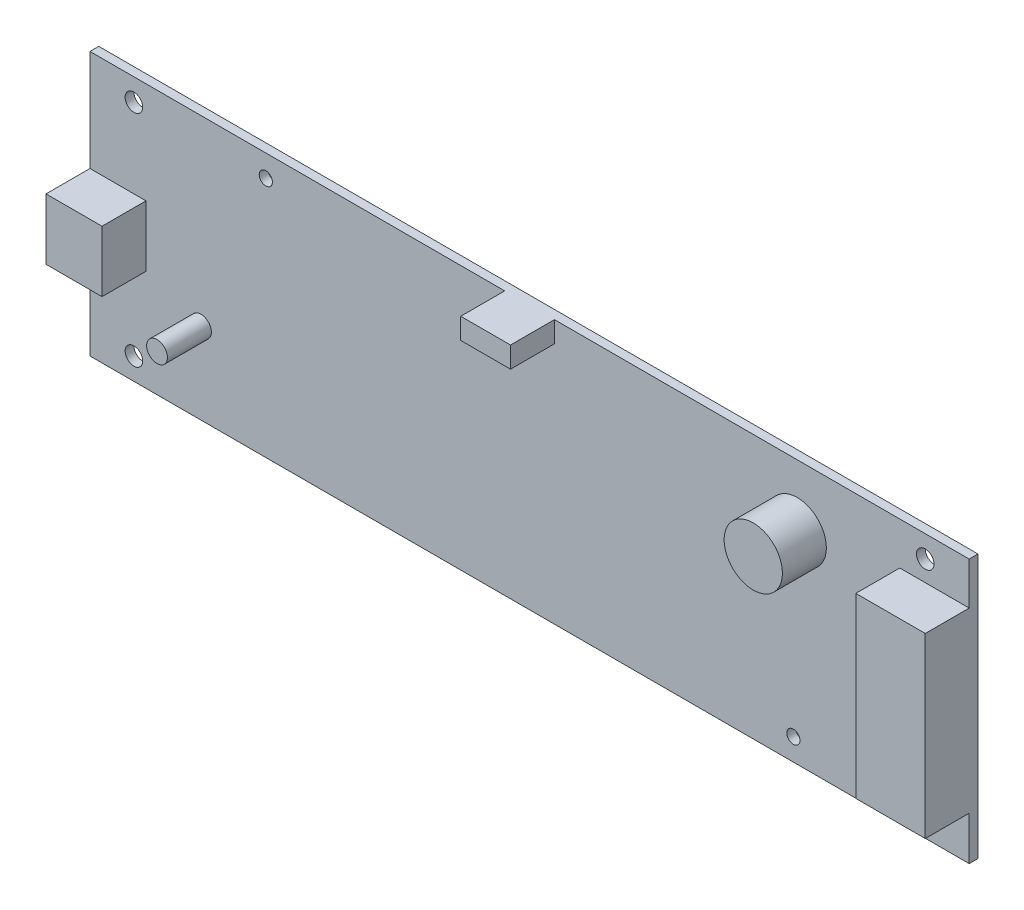
SolidWorks part; units mm, degrees
ref_plane "Front Plane" through (0, 0, 0) normal (0, 0, 1) x (1, 0, 0)
ref_plane "Top Plane" through (0, 0, 0) normal (0, 1, 0) x (1, 0, 0)
ref_plane "Right Plane" through (0, 0, 0) normal (1, 0, 0) x (0, 0, -1)
other "Configuration Table"
sketch "Sketch1" plane through (0, 0, 0) normal (0, 0, 1) x (1, 0, 0)
  line L1 (-50, 15) -> (50, 15)
  line L2 (-50, 15) -> (-50, -15)
  line L3 (-50, -15) -> (50, -15)
  line L4 (50, 15) -> (50, -15)
  line L5 (-50, 15) -> (50, -15) construction
  line L6 (-50, -15) -> (50, 15) construction
  line L7 (-45, 12.5) -> (45, 12.5) construction
  line L8 (-45, 12.5) -> (-45, -12.5) construction
  line L9 (-45, -12.5) -> (45, -12.5) construction
  line L10 (45, 12.5) -> (45, -12.5) construction
  line L11 (-45, 12.5) -> (45, -12.5) construction
  line L12 (-45, -12.5) -> (45, 12.5) construction
  circle A0 centre (-45, -12.5) radius 1
  circle A1 centre (-45, 12.5) radius 1
  circle A2 centre (45, 12.5) radius 1
  circle A3 centre (45, -12.5) radius 1
  point P0 (0, 0)
  point P6 (0, 0)
  dimension "D5" = 2
  dimension "D1" = 100
  dimension "D2" = 30
  dimension "D3" = 25
  dimension "D4" = 90
extrude "Boss-Extrude1" add sketch "Sketch1" along normal blind 1
sketch "Sketch2" plane through (0, 0, 1) normal (0, 0, 1) x (1, 0, 0)
  line L0 (50, -15) -> (50, 15) construction
  line L1 (42.1029, 10.1733) -> (50, 10.1733)
  line L2 (42.1029, 10.1733) -> (42.1029, -10.0282)
  line L3 (42.1029, -10.0282) -> (50, -10.0282)
  line L4 (50, 10.1733) -> (50, -10.0282)
  line L5 (42.1029, 10.1733) -> (50, -10.0282) construction
  line L6 (42.1029, -10.0282) -> (50, 10.1733) construction
  line L7 (50, 15) -> (-50, 15) construction
  line L8 (-2.8295, 12.6173) -> (2.8295, 12.6173)
  line L9 (-2.8295, 12.6173) -> (-2.8295, 15)
  line L10 (-2.8295, 15) -> (2.8295, 15)
  line L11 (2.8295, 12.6173) -> (2.8295, 15)
  line L12 (-2.8295, 12.6173) -> (2.8295, 15) construction
  line L13 (-2.8295, 15) -> (2.8295, 12.6173) construction
  line L14 (-50, 15) -> (-50, -15) construction
  line L15 (-43.6289, -3.4697) -> (-50, -3.4697)
  line L16 (-43.6289, -3.4697) -> (-43.6289, 3.4697)
  line L17 (-43.6289, 3.4697) -> (-50, 3.4697)
  line L18 (-50, -3.4697) -> (-50, 3.4697)
  line L19 (-43.6289, -3.4697) -> (-50, 3.4697) construction
  line L20 (-43.6289, 3.4697) -> (-50, -3.4697) construction
  circle A0 centre (30.4404, 7.9743) radius 3.3121
  circle A1 centre (-37.3722, -5.7496) radius 1.1827
  point P0 (46.0515, 0.0726)
  point P9 (-46.8145, 0)
  point P10 (0, 13.8087)
extrude "Boss-Extrude2" add sketch "Sketch2" along normal blind 5
sketch "Sketch3" plane through (0, 0, 0) normal (0, 0, -1) x (-1, 0, 0)
  line L0 (-50, -7) -> (50, -7) construction
  line L1 (-50, -15) -> (-50, 15) construction
  line L2 (50, 15) -> (50, -15) construction
  line L3 (0, 0) -> (0, 15) construction
  line L4 (-15, -4.5) -> (-10, -4.5)
  line L5 (-15, -4.5) -> (-15, -9.5)
  line L6 (-15, -9.5) -> (-10, -9.5)
  line L7 (-10, -4.5) -> (-10, -9.5)
  line L8 (-15, -4.5) -> (-10, -9.5) construction
  line L9 (-15, -9.5) -> (-10, -4.5) construction
  line L10 (-40, -4.5) -> (-35, -4.5)
  line L11 (-40, -4.5) -> (-40, -9.5)
  line L12 (-40, -9.5) -> (-35, -9.5)
  line L13 (-35, -4.5) -> (-35, -9.5)
  line L14 (-40, -4.5) -> (-35, -9.5) construction
  line L15 (-40, -9.5) -> (-35, -4.5) construction
  line L16 (-50, 15) -> (50, 15) construction
  line L17 (50, -15) -> (-50, -15) construction
  line L18 (40, -4.5) -> (35, -4.5)
  line L19 (40, -4.5) -> (40, -9.5)
  line L20 (40, -9.5) -> (35, -9.5)
  line L21 (35, -4.5) -> (35, -9.5)
  line L22 (15, -4.5) -> (15, -9.5)
  line L23 (15, -4.5) -> (10, -4.5)
  line L24 (10, -4.5) -> (10, -9.5)
  line L25 (15, -9.5) -> (10, -9.5)
  point P6 (-12.5, -7)
  point P11 (-37.5, -7)
  dimension "D1" = 5
  dimension "D2" = 5
  dimension "D3" = 5
  dimension "D4" = 5
  dimension "D5" = 25
  dimension "D6" = 12.5
  dimension "D7" = 8
extrude "Boss-Extrude3" add sketch "Sketch3" along normal blind 1
sketch "Sketch4" plane through (0, 0, -1) normal (0, 0, -1) x (-1, 0, 0)
  circle A0 centre (-37.5, -7) radius 1
  circle A1 centre (-12.5, -7) radius 1
  circle A2 centre (12.5, -7) radius 1
  circle A3 centre (37.5, -7) radius 1
  dimension "D1" = 2
extrude "Boss-Extrude4" add sketch "Sketch4" along normal blind 1
sketch "Sketch5" plane through (0, 0, 1) normal (0, 0, 1) x (1, 0, 0)
  circle A0 centre (30, -12.5) radius 0.75
  circle A1 centre (-30, 12.5) radius 0.75
  circle A2 centre (-45, 12.5) radius 1 construction
  circle A3 centre (45, -12.5) radius 1 construction
  dimension "D1" = 1.5
  dimension "D2" = 15
  dimension "D3" = 1.5
  dimension "D4" = 15
extrude "Cut-Extrude1" cut sketch "Sketch5" against normal blind 10
